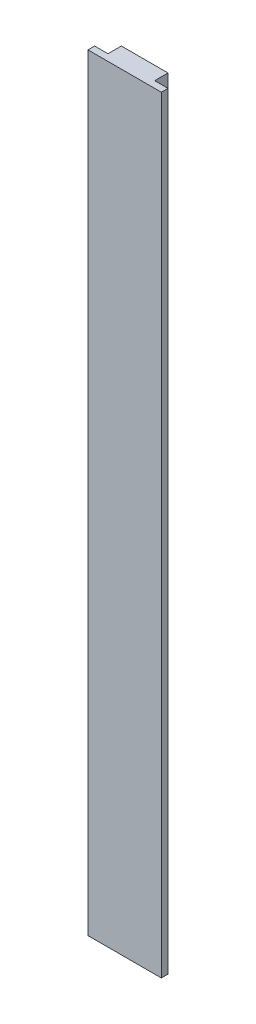
SolidWorks part; units mm, degrees
ref_plane "Front Plane" through (0, 0, 0) normal (0, 0, 1) x (1, 0, 0)
ref_plane "Top Plane" through (0, 0, 0) normal (0, 1, 0) x (1, 0, 0)
ref_plane "Right Plane" through (0, 0, 0) normal (1, 0, 0) x (0, 0, -1)
sketch "Sketch1" plane through (0, 0, 0) normal (0, 1, 0) x (1, 0, 0)
  line L0 (-70, 10) -> (-70, 50)
  line L1 (-110, 10) -> (-70, 10)
  line L2 (-110, 10) -> (-110, -10)
  line L3 (-110, -10) -> (110, -10)
  line L4 (110, 10) -> (110, -10)
  line L5 (-110, 10) -> (110, -10) construction
  line L6 (-110, -10) -> (110, 10) construction
  line L7 (-70, 50) -> (70, 50)
  line L8 (70, 50) -> (70, 10)
  line L9 (70, 10) -> (110, 10)
  point P0 (0, 0)
  dimension "D1" = 220
  dimension "D2" = 20
  dimension "D3" = 40
  dimension "D4" = 40
  dimension "D5" = 40
extrude "Boss-Extrude1" add sketch "Sketch1" along normal blind 2300
hole_wizard "Tap Drill for M10 Tap1" positions "Sketch5" profile "Sketch3" hole size "M10" standard "GB"
sketch "Sketch5" plane through (70, 0, 0) normal (1, 0, 0) x (0, 0, -1)
  line L0 (10, 2300) -> (50, 2300) construction
  line L1 (50, 2300) -> (50, 0) construction
  point P0 (30, 2185)
  dimension "D1" = 115
  dimension "D2" = 20
sketch "Sketch3" plane through (70, 2185, -30) normal (0, 1, 0) x (0, 0, -1)
  line L0 (0, 0) -> (0, 27.5537)
  line L1 (0, 27.5537) -> (4.25, 25)
  line L2 (4.25, 25) -> (4.25, 0.021)
  line L3 (4.25, 0.021) -> (4.275, 0)
  line L5 (4.275, 0) -> (0, 0)
  line L6 (-4.25, 0.021) -> (-4.275, 0) construction
  line L10 (0, 27.5537) -> (-4.25, 25) construction
  line L11 (0, -6.35) -> (0, 107.95) construction
  dimension "孔直径" = 8.5
  dimension "孔深度" = 25
  dimension "近端锥形沉头孔直径" = 8.55
  dimension "近端锥形沉头孔角度" = 100
  dimension "导头角度" = 118
pattern_linear "LPattern1" count 10 spacing 230 along (0, -1, 0) of "Tap Drill for M10 Tap1"
ref_plane "Plane5" through (0, 0, 0) normal (1, 0, 0) x (0, 0, -1)
mirror "Mirror1" about plane through (0, 0, 0) normal (1, 0, 0) of "LPattern1", "Tap Drill for M10 Tap1"
